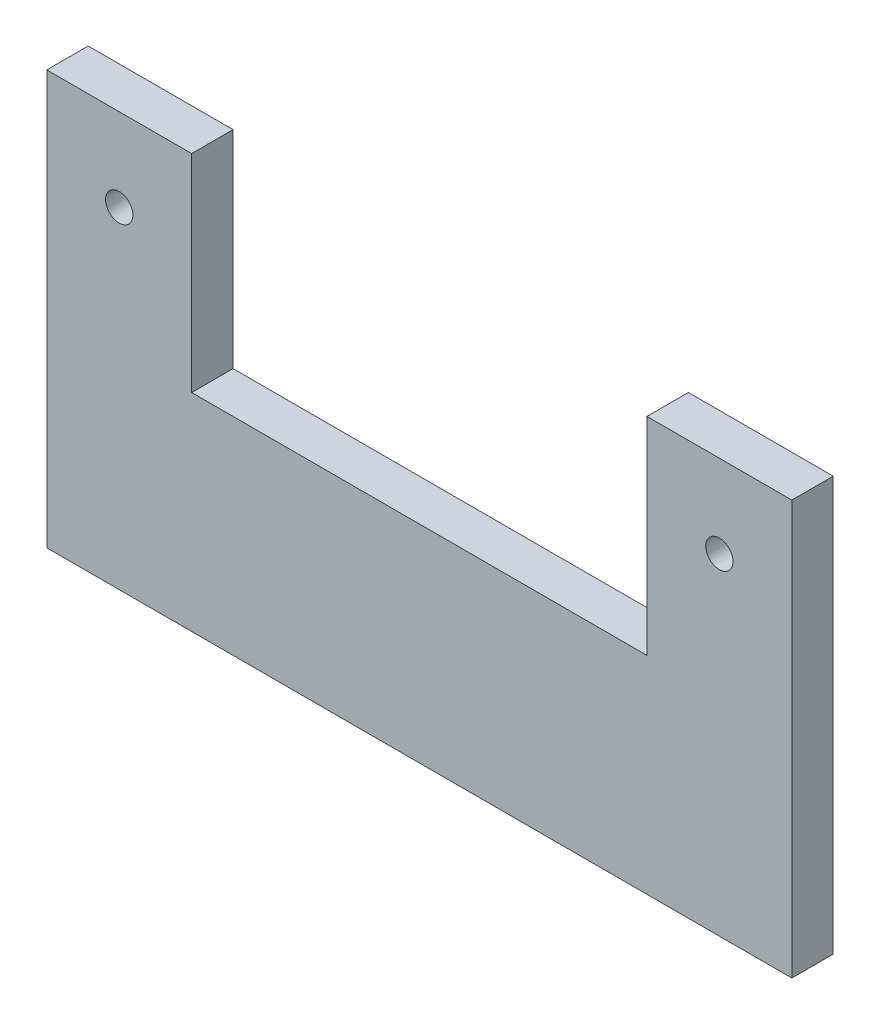
from build123d import *

# Parameters (mm, degrees)
SKETCH_1_W          = 180
SKETCH_1_H          = 100
EXTRUDE_1_DEPTH     = 10
CUT_EXTRUDE_1_REACH = 105.441
SKETCH_2_W          = 110
SKETCH_2_H          = 100
HOLE_WIZARD_M6_1_D  = 6.6


with BuildPart() as part:
    # 草图1 → 凸台-拉伸1 (new body)
    with BuildSketch(Plane.XY):
        Rectangle(SKETCH_1_W, SKETCH_1_H)
    extrude(amount=EXTRUDE_1_DEPTH)

    # 草图2 → 切除-拉伸1 (cut, up to next)
    with BuildSketch(Plane.XY.offset(10), mode=Mode.PRIVATE) as cut_extrude_1_sk1:
        with Locations((0, 50)):
            Rectangle(SKETCH_2_W, SKETCH_2_H)
    cut_extrude_1_tool1 = extrude(cut_extrude_1_sk1.sketch, amount=-CUT_EXTRUDE_1_REACH, mode=Mode.PRIVATE) & part.part
    add(cut_extrude_1_tool1.solids().sort_by_distance((0, 50, 10))[0], mode=Mode.SUBTRACT)

    # M6 间隙孔1 (through all)
    with Locations(Plane(origin=(0, 0, 0), x_dir=(-1, 0, 0), z_dir=(0, 0, -1))):
        with Locations((-72.5, 30), (72.5, 30)):
            Hole(HOLE_WIZARD_M6_1_D / 2)


solid = part.part
